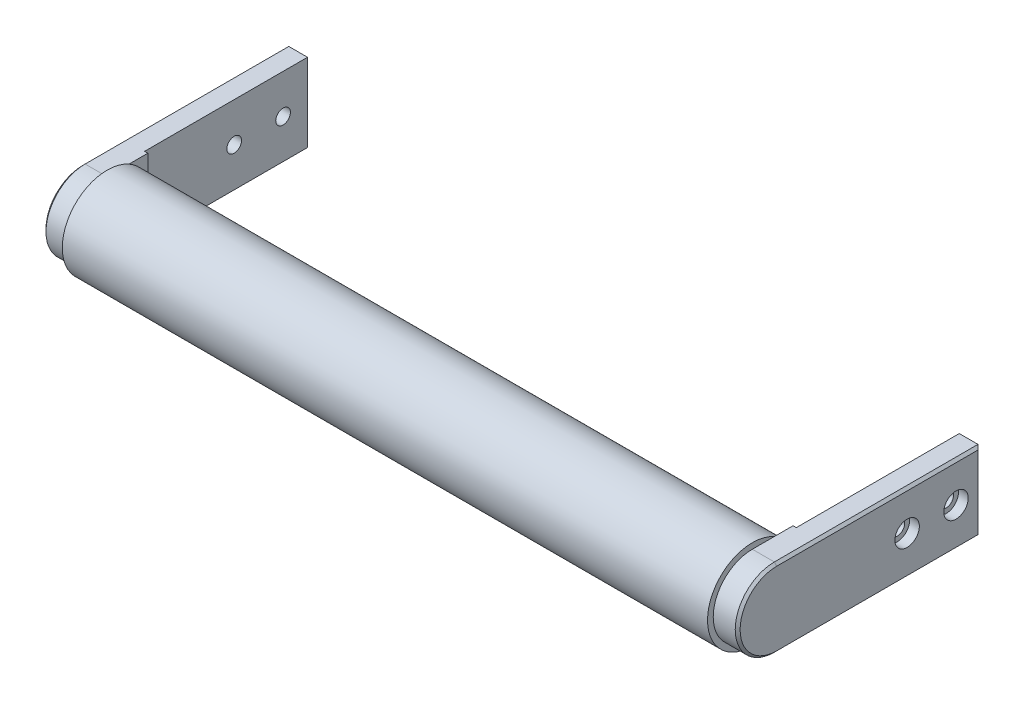
from build123d import *

# Parameters (mm, degrees)
EXTRUDE_1_DEPTH            = 15
SKETCH_2_R                 = 27.5
EXTRUDE_2_DEPTH            = 396
HOLE_WIZARD_1_D            = 9
HOLE_WIZARD_1_CBORE_D      = 15
HOLE_WIZARD_1_CBORE_DEPTH  = 6
CHAMFER_1_SIZE             = 1.5
CHAMFER_1_OF_MIRROR_1_SIZE = 1.5
SKETCH_5_W                 = 2
SKETCH_5_H                 = 100
CUT_EXTRUDE_1_DEPTH        = 424.878815229


with BuildPart() as part:
    # 草图1 → 凸台-拉伸1 (new body)
    with BuildSketch(Plane(origin=(0, 0, 0), x_dir=(0, 0, -1), z_dir=(1, 0, 0))):
        with BuildLine():
            Line((-62.5, 24), (62.5, 24))
            Line((62.5, 24), (62.5, -24))
            Line((62.5, -24), (-62.5, -24))
            ThreePointArc((-62.5, -24), (-86.5, 0), (-62.5, 24))
        make_face()
    extrude_1 = extrude(amount=EXTRUDE_1_DEPTH)

    # 草图2 → 凸台-拉伸2 (add)
    with BuildSketch(Plane.ZY):
        with Locations(Location((62.5, 0, 0), (0, 0, 240.777129706))):
            Circle(SKETCH_2_R)
    extrude(amount=EXTRUDE_2_DEPTH)

    # 打孔尺寸(%根据)内六角花形圆柱头螺钉1 (through all)
    with Locations(Plane(origin=(15, 0, 0), x_dir=(0, 0, -1), z_dir=(1, 0, 0))):
        with Locations((17.5, 0), (47.5, 0)):
            hole_wizard_1 = CounterBoreHole(HOLE_WIZARD_1_D / 2, HOLE_WIZARD_1_CBORE_D / 2, HOLE_WIZARD_1_CBORE_DEPTH)

    # 倒角1
    chamfer_1_edges = [part.edges().sort_by_distance(p)[0] for p in [
        (15, 0, 86.5),
        (15, -24, 0),
        (15, 0, -62.5),
        (15, 24, 0),
    ]]
    chamfer(chamfer_1_edges, length=CHAMFER_1_SIZE)

    # 镜向1: 凸台-拉伸1, 打孔尺寸(%根据)内六角花形圆柱头螺钉1 across plane
    add(extrude_1.mirror(Plane.ZY.offset(198)))
    add(hole_wizard_1.mirror(Plane.ZY.offset(198)), mode=Mode.SUBTRACT)

    # 倒角1 of 镜向1
    chamfer_1_of_mirror_1_edges = [part.edges().sort_by_distance(p)[0] for p in [
        (-411, 0, 86.5),
        (-411, -24, 0),
        (-411, 0, -62.5),
        (-411, 24, 0),
    ]]
    chamfer(chamfer_1_of_mirror_1_edges, length=CHAMFER_1_OF_MIRROR_1_SIZE)

    # 草图5 → 切除-拉伸1 (cut, through all)
    with BuildSketch(Plane(origin=(0, 24, 0), x_dir=(1, 0, 0), z_dir=(0, 1, 0))):
        with Locations((-397, 12.5)):
            Rectangle(SKETCH_5_W, SKETCH_5_H)
        with Locations((1, 12.5)):
            Rectangle(SKETCH_5_W, SKETCH_5_H)
    extrude(amount=-CUT_EXTRUDE_1_DEPTH, mode=Mode.SUBTRACT)


solid = part.part
